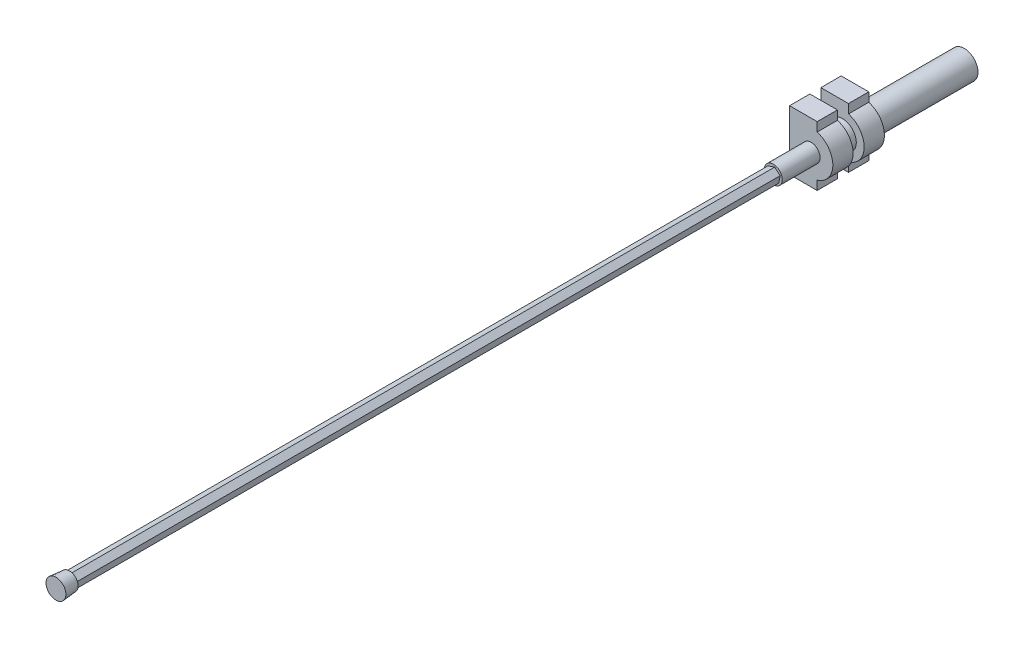
from build123d import *

# Parameters (mm, degrees)
SKETCH1_R           = 46.2
BOSS_EXTRUDE1_DEPTH = 445
SKETCH2_R           = 30
BOSS_EXTRUDE2_DEPTH = 195
BOSS_EXTRUDE3_DEPTH = 2360
BOSS_EXTRUDE4_DEPTH = 68
BOSS_EXTRUDE5_DEPTH = 68


with BuildPart() as part:
    # Sketch1 → Boss-Extrude1 (new body)
    with BuildSketch(Plane.XY):
        Circle(SKETCH1_R)
    extrude(amount=BOSS_EXTRUDE1_DEPTH)

    # Sketch2 → Boss-Extrude2 (add)
    with BuildSketch(Plane.XY.offset(445)):
        Circle(SKETCH2_R)
    extrude(amount=BOSS_EXTRUDE2_DEPTH)

    # Sketch3 → Boss-Extrude3 (add)
    with BuildSketch(Plane.XY.offset(640)):
        Polygon((18.341892461, -15.861115375), (22.907075078, 7.953987137), (4.565182616, 23.815102512), (-18.341892461, 15.861115375), (-22.907075078, -7.953987137), (-4.565182616, -23.815102512), align=None)
    extrude(amount=BOSS_EXTRUDE3_DEPTH)

    # Sketch4 → Revolve1 (revolve)
    with BuildSketch(Plane(origin=(0, 0, 0), x_dir=(1, 0, 0), z_dir=(0, 1, 0)), mode=Mode.PRIVATE) as revolve1_sk:
        Polygon((29.4, -3000), (0, -3000), (0, -3045), (33.3, -3045), align=None)
    revolve(revolve1_sk.sketch.rotate(Axis((0, 0, 0), (0, 0, 1)), 180), axis=Axis((0, 0, 0), (0, 0, 1)))

    # Sketch5 → Boss-Extrude4 (add)
    with BuildSketch(Plane.XY.offset(445)):
        with BuildLine():
            Line((0, 100), (-72.5, 100))
            Line((-72.5, 100), (-72.5, -100))
            Line((-72.5, -100), (0, -100))
            Line((0, -100), (20, -100))
            Line((20, -100), (20, -69.686799324))
            ThreePointArc((20, -69.686799324), (72.5, 0), (20, 69.686799324))
            Line((20, 69.686799324), (20, 100))
            Line((20, 100), (0, 100))
        make_face()
    extrude(amount=BOSS_EXTRUDE4_DEPTH)

    # Sketch6 → Boss-Extrude5 (add)
    with BuildSketch(Plane.XY.offset(340)):
        with BuildLine():
            Line((20, 100), (-72.5, 100))
            Line((-72.5, 100), (-72.5, -100))
            Line((-72.5, -100), (20, -100))
            Line((20, -100), (20, -69.686799324))
            ThreePointArc((20, -69.686799324), (72.5, 0), (20, 69.686799324))
            Line((20, 69.686799324), (20, 100))
        make_face()
    extrude(amount=BOSS_EXTRUDE5_DEPTH)


solid = part.part
